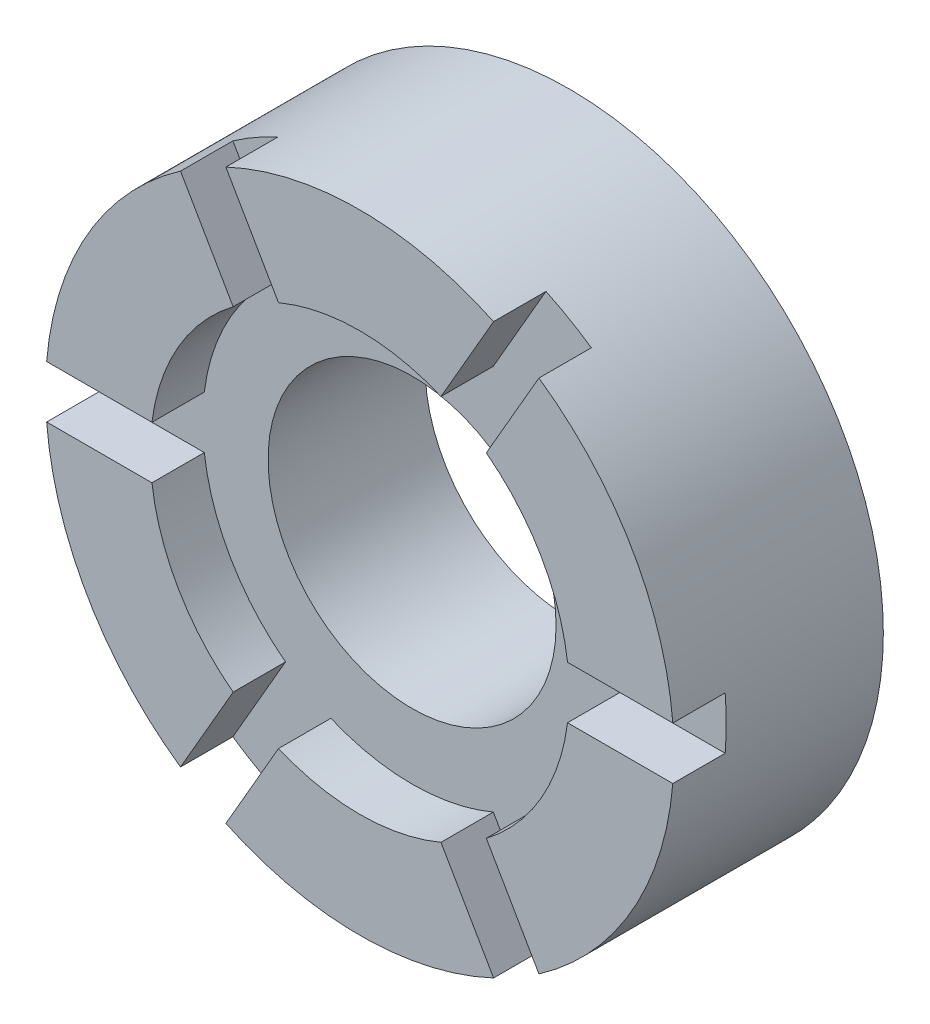
SolidWorks part; units mm, degrees
ref_plane "前视基准面" through (0, 0, 0) normal (0, 0, 1) x (1, 0, 0)
ref_plane "上视基准面" through (0, 0, 0) normal (0, 1, 0) x (1, 0, 0)
ref_plane "右视基准面" through (0, 0, 0) normal (1, 0, 0) x (0, 0, -1)
other "Configuration Table"
sketch "草图1" plane through (0, 0, 0) normal (0, 0, 1) x (1, 0, 0)
  circle A0 centre (0, 0) radius 60
  dimension "D1" = 120
extrude "凸台-拉伸1" add sketch "草图1" along normal blind 40
sketch "草图2" plane through (0, 0, 40) normal (0, 0, 1) x (1, 0, 0)
  circle A0 centre (0, 0) radius 40
  dimension "D1" = 80
extrude "切除-拉伸1" cut sketch "草图2" against normal blind 10
sketch "草图3" plane through (0, 0, 30) normal (0, 0, 1) x (1, 0, 0)
  circle A0 centre (0, 0) radius 27.5
  dimension "D1" = 55
extrude "切除-拉伸2" cut sketch "草图3" against normal up to next
sketch "草图4" plane through (0, 0, 30) normal (0, 0, 1) x (1, 0, 0)
  line L1 (-75, -5) -> (75, -5)
  line L2 (-75, -5) -> (-75, 5)
  line L3 (-75, 5) -> (75, 5)
  line L4 (75, -5) -> (75, 5)
  line L5 (0, 5) -> (0, -5) construction
  line L6 (-75, 0) -> (75, 0) construction
  point P0 (0, 0)
  dimension "D1" = 10
  dimension "D2" = 150
extrude "切除-拉伸3" cut sketch "草图4" along normal up to next
pattern_circular "阵列(圆周)1" count 3 over 360 about axis through (0, 0, 0) along (0, 0, 1) of "切除-拉伸3"
